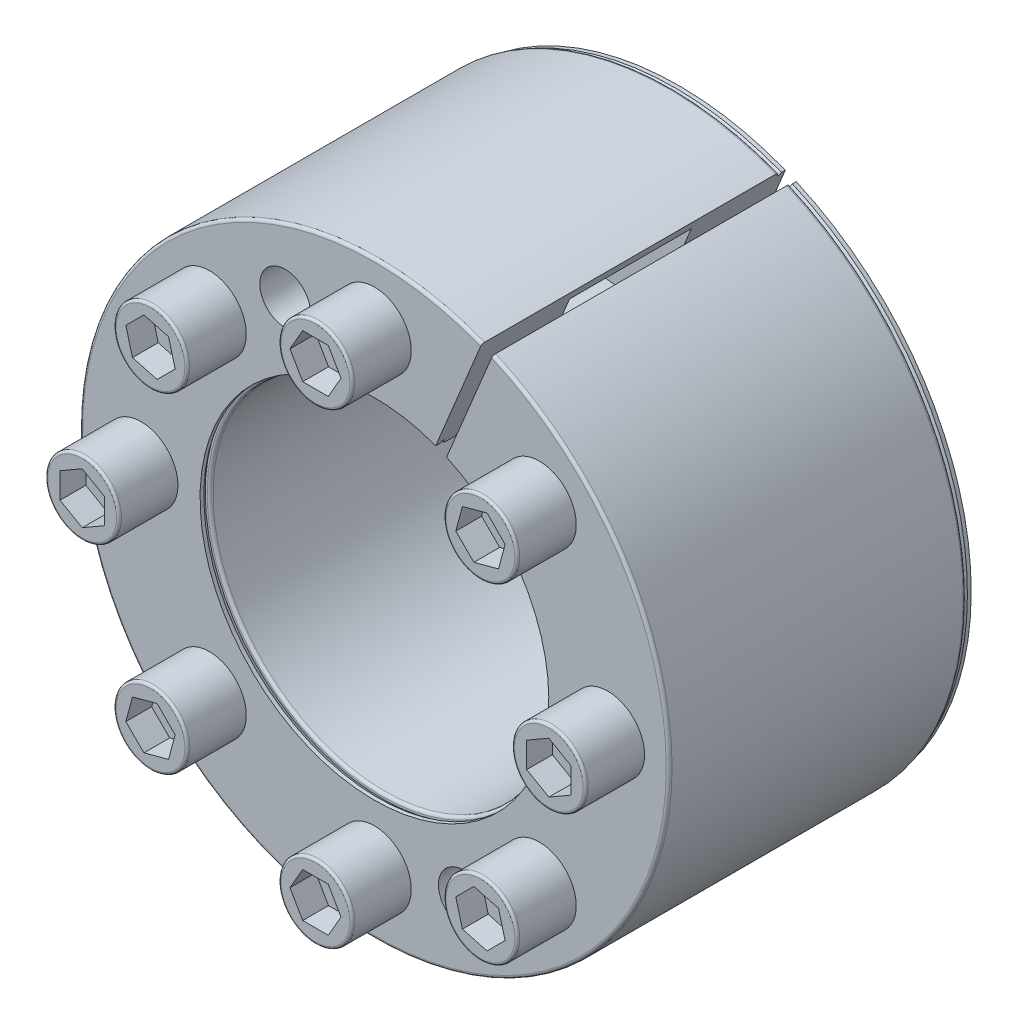
SolidWorks part; units mm, degrees
ref_plane "Front Plane" through (0, 0, 0) normal (0, 0, 1) x (1, 0, 0)
ref_plane "Top Plane" through (0, 0, 0) normal (0, 1, 0) x (1, 0, 0)
ref_plane "Right Plane" through (0, 0, 0) normal (1, 0, 0) x (0, 0, -1)
sketch "Sketch1" plane through (0, 0, 0) normal (1, 0, 0) x (0, 0, -1)
  line L0 (0, 0) -> (31, 0) construction
  line L1 (31, 23.75) -> (-6, 23.75) construction
  line L2 (0, 30) -> (31, 30)
  line L3 (0, 30) -> (0, 17.5)
  line L4 (0, 17.5) -> (31, 17.5)
  line L5 (31, 30) -> (31, 17.5)
  line L6 (15.5, 30) -> (15.5, 17.5) construction
  line L7 (0.775, 30) -> (0.775, 29.5)
  line L8 (0, 29.5) -> (0.775, 29.5)
  line L9 (0, 26.75) -> (31, 26.75)
  line L10 (26.35, 26.75) -> (26.35, 23.75)
  line L11 (31, 26.75) -> (39, 26.75)
  line L13 (9.3, 29.0625) -> (21.7, 29.0625)
  line L14 (9.3, 29.0625) -> (9.3, 18.4375)
  line L15 (9.3, 18.4375) -> (21.7, 18.4375)
  line L16 (21.7, 29.0625) -> (21.7, 18.4375)
  point P16 (26.35, 26.75)
  point P17 (0, 23.75)
  point P25 (15.5, 29.0625)
  point P26 (21.7, 23.75)
  dimension "D1" = 12.4
  dimension "(d)" = 35
  dimension "D2" = 11.5
  dimension "D" = 60
  dimension "L" = 37
  dimension "L1" = 31
  dimension "L2" = 29.45
  dimension "D3" = 4.65
  dimension "(d1)" = 6
  dimension "D4" = 10.625
  dimension "n" = 8
sketch "Sketch2" plane through (0, 0, 0) normal (1, 0, 0) x (0, 0, -1)
  line L0 (0, 17.5) -> (31, 17.5) construction
  line L1 (31, 30) -> (31, 17.5) construction
  line L2 (0, 30) -> (31, 30) construction
  line L3 (0, 30) -> (0, 17.5) construction
  line L4 (0.775, 17.5) -> (31, 17.5)
  line L5 (31, 29.75) -> (31, 17.5)
  line L6 (0, 30) -> (30.225, 30)
  line L7 (0, 30) -> (0, 18)
  line L8 (0.775, 30) -> (0.775, 29.5) construction
  line L9 (0, 29.5) -> (0.775, 29.5) construction
  line L10 (0.775, 30) -> (0.775, 29.5) construction
  line L11 (0, 29.5) -> (0.775, 29.5) construction
  line L12 (31, 23.75) -> (-6, 23.75) construction
  line L13 (31, 23.75) -> (-6, 23.75) construction
  line L14 (0, 18) -> (0.775, 18) construction
  line L15 (0.775, 17.5) -> (0.775, 18)
  line L16 (15.5, 30) -> (15.5, 17.5) construction
  line L17 (15.5, 30) -> (15.5, 17.5) construction
  line L18 (31, 18) -> (30.225, 18) construction
  line L19 (30.225, 17.5) -> (30.225, 18) construction
  line L20 (31, 29.5) -> (30.225, 29.5) construction
  line L21 (30.225, 30) -> (30.225, 29.5)
  line L22 (0, 18) -> (0, 17.75)
  line L23 (31, 29.75) -> (30.6125, 29.75)
  line L24 (30.6125, 29.75) -> (30.225, 29.5)
  line L25 (30.6125, 29.75) -> (30.6125, 29.5) construction
  line L26 (0, 17.75) -> (0.3875, 17.75)
  line L27 (0.3875, 17.75) -> (0.775, 18)
  point P4 (30.225, 29.75)
  point P27 (0.3875, 18)
  point P28 (0.775, 17.75)
revolve "Revolve1" add sketch "Sketch2" angle 360 mid plane about L0
sketch "Sketch7" plane through (0, 0, 0) normal (1, 0, 0) x (0, 0, -1)
  line L0 (21.7, 29.0625) -> (21.7, 18.4375) construction
  line L1 (9.3, 18.4375) -> (21.7, 18.4375) construction
  line L2 (9.3, 29.0625) -> (9.3, 18.4375) construction
  line L3 (9.3, 29.0625) -> (21.7, 29.0625) construction
  line L4 (21.7, 29.0625) -> (21.7, 18.4375)
  line L5 (9.3, 18.4375) -> (21.7, 18.4375)
  line L6 (9.3, 29.0625) -> (9.3, 18.4375)
  line L7 (9.3, 29.0625) -> (21.7, 29.0625)
revolve "Cut-Revolve2" cut sketch "Sketch7" angle 360 mid plane about L0
fillet "Fillet2" radius 0.3 4 edges at (17.5, 0, -0.775) (30, 0, -30.225) (17.5, 0, -31) (30, 0, 0)
sketch "Sketch8" plane through (0, 0, 0) normal (1, 0, 0) x (0, 0, -1)
  line L0 (0, 26.75) -> (31, 26.75) construction
  line L1 (31, 23.75) -> (-6, 23.75) construction
  line L2 (9.3, 26.75) -> (21.7, 26.75)
  line L3 (21.7, 23.75) -> (9.3, 23.75)
  line L4 (9.3, 29.0625) -> (9.3, 18.4375) construction
  line L5 (21.7, 29.0625) -> (21.7, 18.4375) construction
  line L6 (9.3, 26.75) -> (9.3, 23.75)
  line L7 (21.7, 26.75) -> (21.7, 23.75)
revolve "Revolve2" add sketch "Sketch8" angle 360 mid plane about L3
sketch "Screw Sketch1" plane through (-37.0431, 76.0825, 0) normal (0, 0, 1) x (1, 0, 0)
  circle A0 centre (37.0431, -52.3325) radius 3.75
  dimension "D1" = 7.5
extrude "Extrude-Screw (socket head)" add sketch "Screw Sketch1" along normal up to vertex (6 mm away) up to point (0, 23.75, 6)
fillet "Fillet-Screw (socket head)" radius 0.25 1 edges at (3.75, 23.75, 6)
sketch "Screw Sketch2" plane through (0, 82.5, 6) normal (0, 0, 1) x (1, 0, 0)
  line L1 (2.5981, -58.75) -> (1.299, -56.5)
  line L2 (1.299, -56.5) -> (-1.299, -56.5)
  line L3 (-1.299, -56.5) -> (-2.5981, -58.75)
  line L4 (-2.5981, -58.75) -> (-1.299, -61)
  line L5 (-1.299, -61) -> (1.299, -61)
  line L6 (1.299, -61) -> (2.5981, -58.75)
  circle A0 centre (0, -58.75) radius 2.25 construction
  dimension "D1" = 4.5
extrude "Cut-Screw (socket head)" cut sketch "Screw Sketch2" against normal blind 2.625
sketch "Sketch5" plane through (0, 0, 0) normal (1, 0, 0) x (0, 0, -1)
  line L0 (26.35, 26.75) -> (26.35, 23.75) construction
  line L1 (0, 26.75) -> (31, 26.75) construction
  line L2 (31, 23.75) -> (-6, 23.75) construction
  line L3 (31, 30) -> (31, 17.5) construction
  line L4 (26.35, 26.75) -> (26.35, 23.75)
  line L5 (26.35, 26.75) -> (31, 26.75)
  line L6 (31, 23.75) -> (26.35, 23.75)
  line L7 (31, 26.75) -> (31, 23.75)
revolve "Cut-Revolve1" cut sketch "Sketch5" angle 360 mid plane about L6
cosmetic thread "Cosmetic Thread1" parameters "D2"=6.1
pattern_circular "CirPattern1" count 8 over 360 about axis through (0, 0, 0) along (0, 0, 1) of "Cut-Screw (socket head)", "Fillet-Screw (socket head)", "Extrude-Screw (socket head)", "Cut-Revolve1", "Revolve2"
sketch "Sketch6" plane through (0, 0, 0) normal (0, 0, 1) x (1, 0, 0)
  line L0 (0, 30) -> (0, -30) construction
  line L1 (0, 0) -> (11.4805, 27.7164) construction
  line L2 (0, 0) -> (-9.0887, 21.9421) construction
  circle A0 centre (0, 0) radius 30 construction
  circle A1 centre (0, 0) radius 23.75 construction
  circle A2 centre (-9.0887, 21.9421) radius 2.5758
  dimension "D3" = 5.1516
  dimension "D1" = 22.5
  dimension "D2" = 22.5
extrude "Cut-Extrude1" cut sketch "Sketch6" against normal up to vertex (9.3 mm away) up to point (0, 29.0625, -9.3)
cosmetic thread "Cosmetic Thread2" parameters "D2"=5.2516
pattern_circular "CirPattern2" count 2 every 180 about axis through (0, 0, 0) along (0, 0, 1) of "Cut-Extrude1"
sketch "Sketch9" plane through (0, 0, 0) normal (0, 0, 1) x (1, 0, 0)
  line L0 (0, 0) -> (11.4805, 27.7164) construction
  line L1 (0, 0) -> (11.4805, 27.7164)
extrude "Cut-Extrude-Thin1" cut sketch "Sketch9" against normal through all thin thin type mid plane wall 1.2
